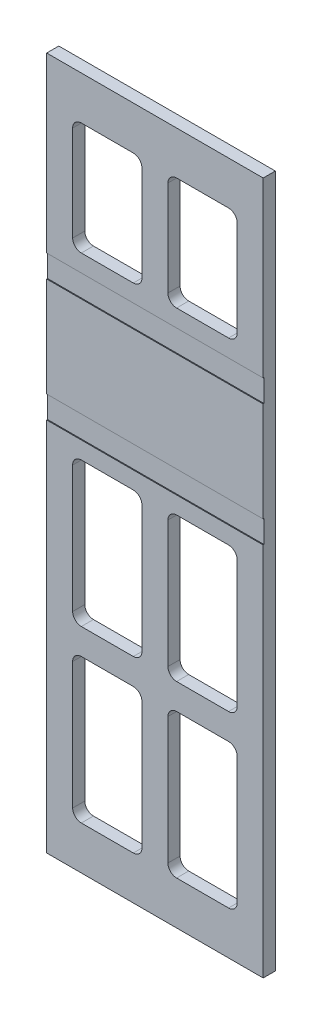
SolidWorks part; units mm, degrees
material "45"
ref_plane "前视基准面" through (0, 0, 0) normal (0, 0, 1) x (1, 0, 0)
ref_plane "上视基准面" through (0, 0, 0) normal (0, 1, 0) x (1, 0, 0)
ref_plane "右视基准面" through (0, 0, 0) normal (1, 0, 0) x (0, 0, -1)
sketch "草图1" plane through (0, 0, 0) normal (0, 0, 1) x (1, 0, 0)
  line L1 (-125, -400) -> (125, -400)
  line L2 (-125, -400) -> (-125, 400)
  line L3 (-125, 400) -> (125, 400)
  line L4 (125, -400) -> (125, 400)
  line L5 (-125, -400) -> (125, 400) construction
  line L6 (-125, 400) -> (125, -400) construction
  point P0 (0, 0)
  dimension "D1" = 250
  dimension "D2" = 800
extrude "凸台-拉伸1" add sketch "草图1" along normal blind 14
sketch "草图2" plane through (0, 0, 14) normal (0, 0, 1) x (1, 0, 0)
  line L0 (-125, 400) -> (-125, -400) construction
  line L1 (-125, 200) -> (125, 200)
  line L2 (-125, 200) -> (-125, 174)
  line L3 (-125, 174) -> (125, 174)
  line L4 (125, 200) -> (125, 174)
  line L5 (125, -400) -> (125, 400) construction
  line L6 (125, 400) -> (-125, 400) construction
  line L7 (-125, 59) -> (125, 59)
  line L8 (-125, 59) -> (-125, 33)
  line L9 (-125, 33) -> (125, 33)
  line L10 (125, 59) -> (125, 33)
  dimension "D1" = 26
  dimension "D2" = 115
  dimension "D3" = 200
extrude "切除-拉伸1" cut sketch "草图2" against normal blind 1
sketch "草图3" plane through (0, 0, 14) normal (0, 0, 1) x (1, 0, 0)
  line L0 (-125, 33) -> (125, 33) construction
  line L1 (-95, -153.5) -> (-15, -153.5)
  line L2 (-95, -153.5) -> (-95, 13)
  line L3 (-95, 13) -> (-15, 13)
  line L4 (-15, -153.5) -> (-15, 13)
  line L5 (-95, -153.5) -> (-15, 13) construction
  line L6 (-95, 13) -> (-15, -153.5) construction
  line L7 (-125, 33) -> (-125, -400) construction
  line L8 (-125, -400) -> (125, -400) construction
  line L9 (-95, -350) -> (-15, -350)
  line L10 (-95, -350) -> (-95, -183.5)
  line L11 (-95, -183.5) -> (-15, -183.5)
  line L12 (-15, -350) -> (-15, -183.5)
  line L13 (-95, -350) -> (-15, -183.5) construction
  line L14 (-95, -183.5) -> (-15, -350) construction
  line L15 (0, 0) -> (0, 33) construction
  line L16 (-125, 33) -> (125, 33) construction
  line L17 (95, -183.5) -> (15, -350) construction
  line L18 (95, -350) -> (15, -183.5) construction
  line L19 (95, 13) -> (15, -153.5) construction
  line L20 (95, -153.5) -> (15, 13) construction
  line L21 (15, -350) -> (15, -183.5)
  line L22 (95, -183.5) -> (15, -183.5)
  line L23 (95, -350) -> (95, -183.5)
  line L24 (95, -350) -> (15, -350)
  line L25 (15, -153.5) -> (15, 13)
  line L26 (95, 13) -> (15, 13)
  line L27 (95, -153.5) -> (95, 13)
  line L28 (95, -153.5) -> (15, -153.5)
  line L29 (125, 400) -> (-125, 400) construction
  line L30 (-95, 220) -> (-15, 220)
  line L31 (-95, 220) -> (-95, 350)
  line L32 (-95, 350) -> (-15, 350)
  line L33 (-15, 220) -> (-15, 350)
  line L34 (-95, 220) -> (-15, 350) construction
  line L35 (-95, 350) -> (-15, 220) construction
  line L36 (15, 220) -> (95, 220)
  line L37 (15, 220) -> (15, 350)
  line L38 (15, 350) -> (95, 350)
  line L39 (95, 220) -> (95, 350)
  line L40 (15, 220) -> (95, 350) construction
  line L41 (15, 350) -> (95, 220) construction
  line L42 (125, 200) -> (-125, 200) construction
  point P0 (-55, -70.25)
  point P10 (-55, -266.75)
  point P29 (55, -266.75)
  point P30 (55, -70.25)
  point P31 (-55, 285)
  point P36 (55, 285)
  dimension "D1" = 20
  dimension "D2" = 30
  dimension "D3" = 15
  dimension "D4" = 30
  dimension "D5" = 50
  dimension "D6" = 50
  dimension "D7" = 20
extrude "切除-拉伸2" cut sketch "草图3" against normal up to next
fillet "圆角1" radius 10 24 edges at (-95, -153.5, 7) (-15, -153.5, 7) (-15, 13, 7) (-95, -183.5, 7) (-95, -350, 7) (-15, -350, 7) (-15, -183.5, 7) (15, -183.5, 7) (15, -350, 7) (95, -350, 7) (95, -183.5, 7) (15, 13, 7) (15, -153.5, 7) (95, -153.5, 7) (95, 13, 7) (-95, 13, 7) (-15, 220, 7) (-95, 220, 7) (-95, 350, 7) (-15, 350, 7) (15, 220, 7) (15, 350, 7) (95, 220, 7) (95, 350, 7)
